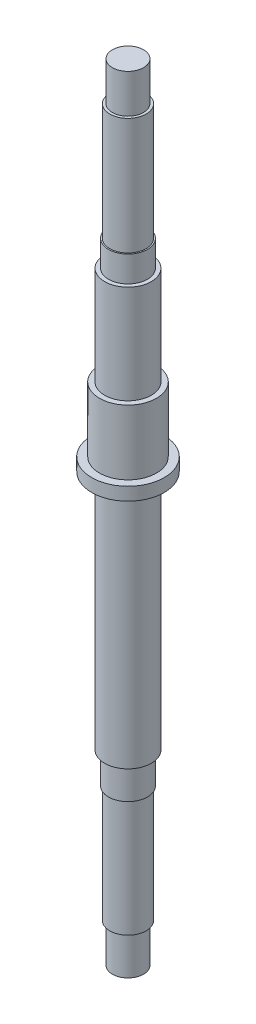
from build123d import *


with BuildPart() as part:
    # Sketch1 → Revolve1 (revolve)
    with BuildSketch(Plane.XY):
        Polygon((0, 303), (-6, 303), (-6, 288), (-7, 288), (-7, 243), (-7.5, 243), (-7.5, 233), (-9, 233), (-9, 195), (-11, 195), (-11, 170), (-14, 170), (-14, 165), (-9, 165), (-9, 72), (-7.5, 72), (-7.5, 60), (-7, 60), (-7, 15), (-6, 15), (-6, 0), (0, 0), align=None)
    revolve(axis=Axis((0, 303, 0), (0, -1, 0)))


solid = part.part
